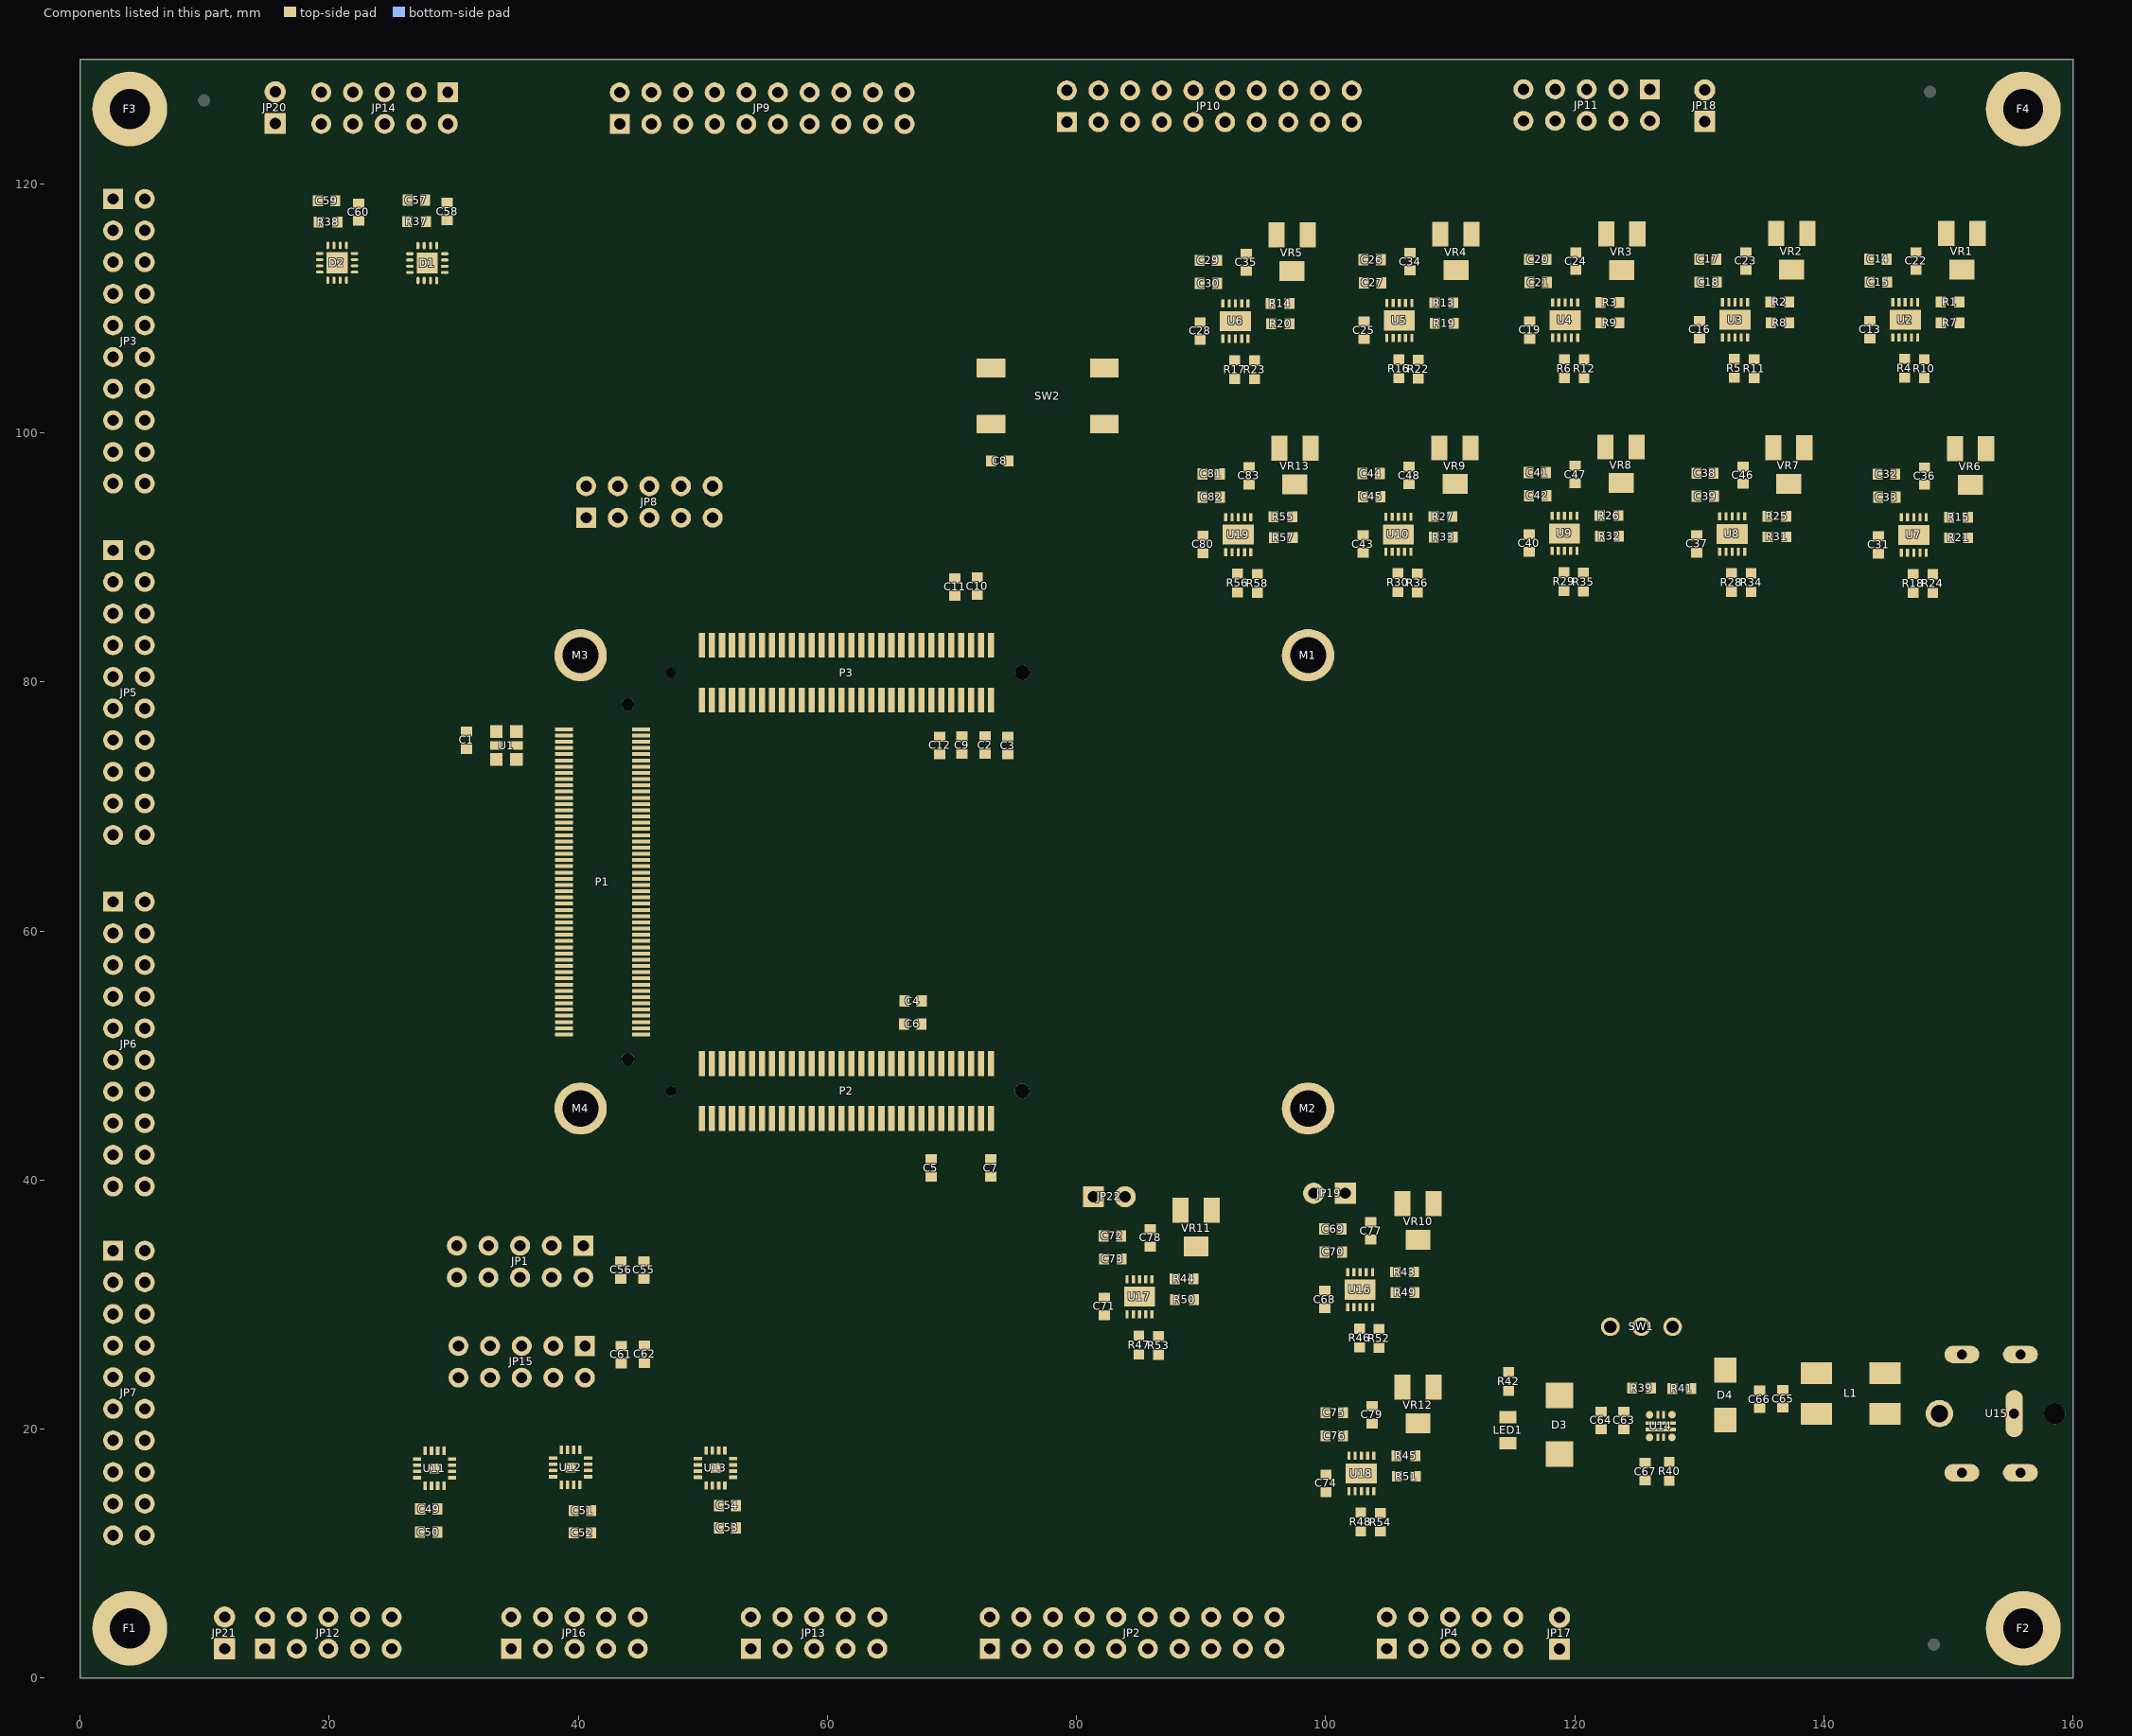
[diagram p0: the components of this part, seen from the top]
# Altium PCB MISC82195.PcbDoc (part 7 of 8)
Units mm, origin at the board's own origin, x right, y up, seen from the top; angles counter-clockwise.
Board outline 160 x 130 mm, 4 copper layers (Top Layer, GND, POWER, Bottom Layer); 214 components, 251 nets, 1068 pads, 1218 vias.

## Polygon pours and split planes (outlines as drawn) (continued)
VCC5VD on Top Layer "Bottom Layer-No Net" (solid, remove dead copper, pour order 1031): 113.081,17.374 113.081,14.199 113.411,13.868 114.071,13.208 115.316,13.208 122.58,13.208 123.038,13.665 123.723,14.351 123.723,16.891 123.723,17.323 124.79,18.39 125.095,18.694 125.095,19.228 125.095,19.38 125.298,19.583 125.527,19.812 125.806,19.812 128.092,19.812 128.143,19.863 128.168,19.888 128.168,19.964 128.168,20.117 128.143,20.142 127.991,20.142 125.552,20.142 125.451,20.244 125.273,20.422 124.333,20.422 120.802,20.422 120.421,20.041 119.736,19.355 118.389,19.355 113.767,19.355 113.411,18.999 113.106,18.694 113.106,17.475
NetC65_2 on Top Layer "Bottom Layer-No Net" (solid, remove dead copper, pour order 1030): 125.679,20.523 125.679,20.371 125.705,20.345 125.73,20.32 125.781,20.32 128.575,20.32 128.651,20.244 128.753,20.142 128.753,19.837 128.753,18.567 128.88,18.44 129.794,17.526 131.521,17.526 139.878,17.526 140.31,17.958 140.716,18.364 140.716,20.091 140.716,21.844 140.462,22.098 140.437,22.123 138.354,22.123 130.734,22.123 130.454,22.403 130.226,22.631 130.226,23.317 130.226,23.647 130.124,23.749 130.073,23.8 129.667,23.8 129.032,23.8 128.956,23.724 128.956,23.546 128.956,21.361 128.6,21.006 128.245,20.65 127.889,20.65 125.705,20.65 125.679,20.625 125.679,20.523
NetL1_2 on Top Layer "Bottom Layer-No Net" (solid, remove dead copper, pour order 1029): 143.561,25.654 143.561,23.749 143.612,23.698 143.84,23.47 144.602,23.47 146.279,23.47 146.634,23.825 147.269,24.46 148.869,24.46 152.248,24.46 152.984,23.724 153.67,23.038 153.67,21.463 153.67,18.313 153.568,18.212 152.857,17.501 150.571,17.501 149.479,17.501 149.098,17.12 148.742,16.764 148.742,15.748 148.742,13.97 149.2,13.513 149.606,13.106 151.105,13.106 156.134,13.106 156.642,13.614 157.226,14.199 157.226,18.948 157.226,28.55 156.439,29.337 156.286,29.489 152.984,29.489 144.932,29.489 144.145,28.702 143.561,28.118 143.561,25.679
NetL1_1 on Top Layer "Bottom Layer-No Net" (solid, remove dead copper, pour order 1028): 143.459,21.336 143.459,18.771 143.688,18.542 143.942,18.288 145.059,18.288 149.809,18.288 150.012,18.491 150.419,18.898 150.419,20.015 150.419,21.844 150.012,22.25 149.86,22.403 148.158,22.403 147.396,22.403 147.142,22.149 145.847,22.149 143.688,22.149 143.561,22.022 143.459,21.92 143.459,21.336
VCC1V8D on Top Layer "Bottom Layer-No Net" (solid, remove dead copper, pour order 1027): 100.99,20.803 100.99,17.863 101.346,17.548 101.371,17.526 101.905,17.526 102.413,17.526 102.464,17.571 102.489,17.593 102.489,17.75 102.489,22.15 102.286,22.33 102.26,22.352 101.93,22.352 101.321,22.352 101.117,22.172 100.99,22.06 100.99,20.826
VCC5VD on Top Layer "Bottom Layer-No Net" (solid, remove dead copper, pour order 1026): 99.212,14.58 99.212,11.582 99.568,11.227 99.974,10.82 100.686,10.82 102.972,10.82 103.124,10.973 103.429,11.278 103.429,11.506 103.429,12.09 103.276,12.243 103.048,12.243 102.21,12.243 102.057,12.395 101.905,12.548 101.905,12.903 101.905,13.894 102.006,13.995 102.133,14.122 102.286,14.122 102.641,14.122 102.768,14.249 102.997,14.478 102.997,14.859 102.997,15.24 102.921,15.316 102.895,15.342 102.794,15.342 99.67,15.342 99.492,15.164 99.212,14.884 99.212,14.554
VCC5VD on Top Layer "Bottom Layer-No Net" (solid, remove dead copper, pour order 1024): 99.111,29.337 99.111,26.34 99.466,25.984 99.873,25.578 100.584,25.578 102.87,25.578 103.022,25.73 103.327,26.035 103.327,26.264 103.327,26.848 103.175,27 102.946,27 102.108,27 101.956,27.153 101.803,27.305 101.803,27.661 101.803,28.651 101.905,28.753 102.032,28.88 102.184,28.88 102.54,28.88 102.667,29.007 102.895,29.235 102.895,29.616 102.895,29.997 102.819,30.074 102.794,30.099 102.692,30.099 99.568,30.099 99.39,29.921 99.111,29.642 99.111,29.312
VCC5VD on Top Layer "Bottom Layer-No Net" (solid, remove dead copper, pour order 1022): 81.407,28.778 81.407,25.781 81.763,25.425 82.169,25.019 82.88,25.019 85.166,25.019 85.319,25.171 85.623,25.476 85.623,25.705 85.623,26.289 85.471,26.441 85.242,26.441 84.404,26.441 84.252,26.594 84.099,26.746 84.099,27.102 84.099,28.092 84.201,28.194 84.328,28.321 84.48,28.321 84.836,28.321 84.963,28.448 85.192,28.677 85.192,29.058 85.192,29.439 85.115,29.515 85.09,29.54 84.988,29.54 81.864,29.54 81.686,29.362 81.407,29.083 81.407,28.753
VCC5VD on Top Layer "Bottom Layer-No Net" (solid, remove dead copper, pour order 1021): 143.561,89.941 143.561,86.944 143.916,86.589 144.323,86.182 145.034,86.182 147.32,86.182 147.472,86.335 147.777,86.639 147.777,86.868 147.777,87.452 147.625,87.605 147.396,87.605 146.558,87.605 146.406,87.757 146.253,87.909 146.253,88.265 146.253,89.256 146.355,89.357 146.482,89.484 146.634,89.484 146.99,89.484 147.117,89.611 147.345,89.84 147.345,90.221 147.345,90.602 147.269,90.678 147.244,90.703 147.142,90.703 144.018,90.703 143.84,90.526 143.561,90.246 143.561,89.916
LDO_6 on Top Layer "Bottom Layer-No Net" (solid, remove dead copper, pour order 1020): 145.339,96.165 145.339,93.224 145.694,92.91 145.72,92.888 146.253,92.888 146.761,92.888 146.812,92.933 146.837,92.955 146.837,93.112 146.837,97.512 146.634,97.691 146.609,97.714 146.279,97.714 145.669,97.714 145.466,97.534 145.339,97.422 145.339,96.187
VCC5VD on Top Layer "Bottom Layer-No Net" (solid, remove dead copper, pour order 1019): 128.981,90.018 128.981,87.02 129.337,86.665 129.743,86.258 130.454,86.258 132.74,86.258 132.893,86.411 133.198,86.716 133.198,86.944 133.198,87.528 133.045,87.681 132.817,87.681 131.978,87.681 131.826,87.833 131.674,87.986 131.674,88.341 131.674,89.332 131.775,89.433 131.902,89.56 132.055,89.56 132.41,89.56 132.537,89.687 132.766,89.916 132.766,90.297 132.766,90.678 132.69,90.754 132.664,90.78 132.563,90.78 129.438,90.78 129.261,90.602 128.981,90.322 128.981,89.992
LDO_7 on Top Layer "Bottom Layer-No Net" (solid, remove dead copper, pour order 1018): 130.759,96.241 130.759,93.301 131.115,92.986 131.14,92.964 131.674,92.964 132.182,92.964 132.232,93.009 132.258,93.031 132.258,93.188 132.258,97.588 132.055,97.768 132.029,97.79 131.699,97.79 131.089,97.79 130.886,97.61 130.759,97.498 130.759,96.264
VCC5VD on Top Layer "Bottom Layer-No Net" (solid, remove dead copper, pour order 1017): 115.519,90.068 115.519,87.071 115.875,86.716 116.281,86.309 116.992,86.309 119.278,86.309 119.431,86.462 119.736,86.766 119.736,86.995 119.736,87.579 119.583,87.732 119.355,87.732 118.516,87.732 118.364,87.884 118.212,88.036 118.212,88.392 118.212,89.383 118.313,89.484 118.44,89.611 118.593,89.611 118.948,89.611 119.075,89.738 119.304,89.967 119.304,90.348 119.304,90.729 119.228,90.805 119.202,90.83 119.101,90.83 115.976,90.83 115.799,90.653 115.519,90.373 115.519,90.043
LDO_8 on Top Layer "Bottom Layer-No Net" (solid, remove dead copper, pour order 1016): 117.297,96.292 117.297,93.351 117.653,93.037 117.678,93.015 118.212,93.015 118.72,93.015 118.77,93.06 118.796,93.082 118.796,93.239 118.796,97.639 118.593,97.818 118.567,97.841 118.237,97.841 117.627,97.841 117.424,97.661 117.297,97.549 117.297,96.314
VCC5VD on Top Layer "Bottom Layer-No Net" (solid, remove dead copper, pour order 1015): 102.184,89.992 102.184,86.995 102.54,86.639 102.946,86.233 103.657,86.233 105.943,86.233 106.096,86.385 106.401,86.69 106.401,86.919 106.401,87.503 106.248,87.655 106.02,87.655 105.181,87.655 105.029,87.808 104.877,87.96 104.877,88.316 104.877,89.306 104.978,89.408 105.105,89.535 105.258,89.535 105.613,89.535 105.74,89.662 105.969,89.891 105.969,90.272 105.969,90.653 105.893,90.729 105.867,90.754 105.766,90.754 102.641,90.754 102.464,90.576 102.184,90.297 102.184,89.967
LDO_9 on Top Layer "Bottom Layer-No Net" (solid, remove dead copper, pour order 1014): 103.962,96.216 103.962,93.275 104.318,92.961 104.343,92.939 104.877,92.939 105.385,92.939 105.435,92.983 105.461,93.006 105.461,93.163 105.461,97.563 105.258,97.742 105.232,97.765 104.902,97.765 104.292,97.765 104.089,97.585 103.962,97.473 103.962,96.238
VCC5VD on Top Layer "Bottom Layer-No Net" (solid, remove dead copper, pour order 1013): 89.332,89.967 89.332,86.97 89.687,86.614 90.094,86.208 90.805,86.208 93.091,86.208 93.243,86.36 93.548,86.665 93.548,86.893 93.548,87.478 93.396,87.63 93.167,87.63 92.329,87.63 92.177,87.782 92.024,87.935 92.024,88.29 92.024,89.281 92.126,89.383 92.253,89.51 92.405,89.51 92.761,89.51 92.888,89.637 93.116,89.865 93.116,90.246 93.116,90.627 93.04,90.703 93.015,90.729 92.913,90.729 89.789,90.729 89.611,90.551 89.332,90.272 89.332,89.941
LDO_10 on Top Layer "Bottom Layer-No Net" (solid, remove dead copper, pour order 1012): 91.11,96.19 91.11,93.25 91.465,92.936 91.491,92.913 92.024,92.913 92.532,92.913 92.583,92.958 92.608,92.981 92.608,93.138 92.608,97.537 92.405,97.717 92.38,97.739 92.05,97.739 91.44,97.739 91.237,97.56 91.11,97.447 91.11,96.213
LDO_1 on Top Layer "Bottom Layer-No Net" (solid, remove dead copper, pour order 1011): 144.653,113.437 144.653,110.496 145.009,110.182 145.034,110.16 145.567,110.16 146.075,110.16 146.126,110.205 146.152,110.227 146.152,110.384 146.152,114.784 145.948,114.963 145.923,114.986 145.593,114.986 144.983,114.986 144.78,114.806 144.653,114.694 144.653,113.459
VCC5VD on Top Layer "Bottom Layer-No Net" (solid, remove dead copper, pour order 1010): 142.875,107.213 142.875,104.216 143.231,103.861 143.637,103.454 144.348,103.454 146.634,103.454 146.787,103.607 147.091,103.911 147.091,104.14 147.091,104.724 146.939,104.877 146.71,104.877 145.872,104.877 145.72,105.029 145.567,105.181 145.567,105.537 145.567,106.528 145.669,106.629 145.796,106.756 145.948,106.756 146.304,106.756 146.431,106.883 146.66,107.112 146.66,107.493 146.66,107.874 146.583,107.95 146.558,107.975 146.456,107.975 143.332,107.975 143.154,107.798 142.875,107.518 142.875,107.188
LDO_2 on Top Layer "Bottom Layer-No Net" (solid, remove dead copper, pour order 1009): 130.988,113.437 130.988,110.496 131.343,110.182 131.369,110.16 131.902,110.16 132.41,110.16 132.461,110.205 132.486,110.227 132.486,110.384 132.486,114.784 132.283,114.963 132.258,114.986 131.928,114.986 131.318,114.986 131.115,114.806 130.988,114.694 130.988,113.459
VCC5VD on Top Layer "Bottom Layer-No Net" (solid, remove dead copper, pour order 1008): 129.21,107.213 129.21,104.216 129.565,103.861 129.972,103.454 130.683,103.454 132.969,103.454 133.121,103.607 133.426,103.911 133.426,104.14 133.426,104.724 133.274,104.877 133.045,104.877 132.207,104.877 132.055,105.029 131.902,105.181 131.902,105.537 131.902,106.528 132.004,106.629 132.131,106.756 132.283,106.756 132.639,106.756 132.766,106.883 132.994,107.112 132.994,107.493 132.994,107.874 132.918,107.95 132.893,107.975 132.791,107.975 129.667,107.975 129.489,107.798 129.21,107.518 129.21,107.188
LDO_3 on Top Layer "Bottom Layer-No Net" (solid, remove dead copper, pour order 1007): 117.348,113.412 117.348,110.471 117.704,110.157 117.729,110.134 118.262,110.134 118.77,110.134 118.821,110.179 118.847,110.202 118.847,110.359 118.847,114.758 118.643,114.938 118.618,114.96 118.288,114.96 117.678,114.96 117.475,114.781 117.348,114.669 117.348,113.434
VCC5VD on Top Layer "Bottom Layer-No Net" (solid, remove dead copper, pour order 1006): 115.57,107.188 115.57,104.191 115.926,103.835 116.332,103.429 117.043,103.429 119.329,103.429 119.482,103.581 119.786,103.886 119.786,104.115 119.786,104.699 119.634,104.851 119.405,104.851 118.567,104.851 118.415,105.004 118.262,105.156 118.262,105.512 118.262,106.502 118.364,106.604 118.491,106.731 118.643,106.731 118.999,106.731 119.126,106.858 119.355,107.086 119.355,107.467 119.355,107.848 119.278,107.925 119.253,107.95 119.151,107.95 116.027,107.95 115.849,107.772 115.57,107.493 115.57,107.163
VCC5VD on Top Layer "Bottom Layer-No Net" (solid, remove dead copper, pour order 1005): 102.26,107.163 102.26,104.165 102.616,103.81 103.022,103.403 103.734,103.403 106.02,103.403 106.172,103.556 106.477,103.861 106.477,104.089 106.477,104.673 106.324,104.826 106.096,104.826 105.258,104.826 105.105,104.978 104.953,105.131 104.953,105.486 104.953,106.477 105.054,106.578 105.181,106.705 105.334,106.705 105.689,106.705 105.816,106.832 106.045,107.061 106.045,107.442 106.045,107.823 105.969,107.899 105.943,107.925 105.842,107.925 102.718,107.925 102.54,107.747 102.26,107.467 102.26,107.137
LDO_4 on Top Layer "Bottom Layer-No Net" (solid, remove dead copper, pour order 1004): 104.038,113.386 104.038,110.446 104.394,110.131 104.419,110.109 104.953,110.109 105.461,110.109 105.512,110.154 105.537,110.176 105.537,110.333 105.537,114.733 105.334,114.913 105.308,114.935 104.978,114.935 104.369,114.935 104.165,114.755 104.038,114.643 104.038,113.409
LDO_5 on Top Layer "Bottom Layer-No Net" (solid, remove dead copper, pour order 1003): 90.881,113.335 90.881,110.395 91.237,110.081 91.262,110.058 91.796,110.058 92.304,110.058 92.354,110.103 92.38,110.126 92.38,110.283 92.38,114.682 92.177,114.862 92.151,114.884 91.821,114.884 91.211,114.884 91.008,114.705 90.881,114.592 90.881,113.358
VCC5VD on Top Layer "Bottom Layer-No Net" (solid, remove dead copper, pour order 1002): 89.103,107.112 89.103,104.115 89.459,103.759 89.865,103.353 90.576,103.353 92.862,103.353 93.015,103.505 93.32,103.81 93.32,104.038 93.32,104.623 93.167,104.775 92.939,104.775 92.1,104.775 91.948,104.927 91.796,105.08 91.796,105.435 91.796,106.426 91.897,106.528 92.024,106.655 92.177,106.655 92.532,106.655 92.659,106.782 92.888,107.01 92.888,107.391 92.888,107.772 92.812,107.848 92.786,107.874 92.685,107.874 89.56,107.874 89.383,107.696 89.103,107.417 89.103,107.086
NetJP8_1 on Top Layer "Bottom Layer-No Net" (solid, remove dead copper, pour order 1001): 39.675,93.116 39.675,90.246 40.157,89.764 40.843,89.078 43.231,89.078 46.431,89.078 47.142,88.367 49.505,86.004 49.505,83.058 49.505,82.067 49.555,82.017 49.682,81.89 49.809,81.89 52.476,81.89 52.502,81.915 52.578,81.991 52.578,82.423 52.578,93.116 51.968,93.726 51.664,94.031 50.622,94.031 39.878,94.031 39.776,93.929 39.675,93.828 39.675,93.116
NetJP1_1 on Top Layer "Bottom Layer-No Net" (solid, remove dead copper, pour order 1000): 29.388,35.331 29.388,34.671 29.388,34.265 29.667,33.985 29.921,33.731 31.14,33.731 41.427,33.731 42.443,34.747 45.314,37.617 47.244,37.617 49.327,37.617 50.546,38.837 52.578,40.869 52.578,44.044 52.578,45.847 52.502,45.923 52.426,45.999 51.943,45.999 49.733,45.999 49.657,45.923 49.301,45.568 49.301,44.806 49.301,44.044 48.158,42.901 47.142,41.885 46.101,41.885 45.364,41.885 43.942,40.462 40.284,36.805 34.011,36.805 30.683,36.805 29.413,35.535 29.388,35.509 29.388,35.331
VCC3V3D on Top Layer "Bottom Layer-No Net" (solid, remove dead copper, pour order 1000): 100.66,39.268 100.66,38.735 100.66,37.059 100.762,36.957 100.838,36.881 100.838,36.474 100.838,32.588 101.016,32.41 101.168,32.258 101.625,32.258 102.311,32.258 102.362,32.309 102.413,32.36 102.413,32.537 102.413,37.287 102.591,37.465 102.845,37.719 102.845,38.329 102.845,39.726 102.667,39.903 102.54,40.03 102.133,40.03 100.889,40.03 100.686,39.827 100.66,39.802 100.66,39.294
VCC2V5D on Top Layer "Bottom Layer-No Net" (solid, remove dead copper, pour order 1001): 83.007,38.76 83.007,36.347 83.134,36.22 83.185,36.17 83.185,35.89 83.185,32.004 83.388,31.801 83.464,31.725 83.998,31.725 84.607,31.725 84.658,31.775 84.684,31.801 84.684,31.902 84.684,32.537 84.785,32.639 84.912,32.766 84.912,32.944 84.912,39.243 84.658,39.497 84.531,39.624 84.328,39.624 83.337,39.624 83.134,39.421 83.007,39.294 83.007,38.76
GND on Bottom Layer "Bottom Layer-No Net" (solid, remove dead copper, pour order 1034): -7.925,128.981 -7.925,-4.267 -3.048,-9.144 -0.787,-11.405 6.325,-11.405 161.747,-11.405 165.506,-7.645 172.644,-0.508 172.644,18.237 172.644,132.74 165.887,139.497 160.63,144.755 147.853,144.755 2.184,144.755 -5.309,137.262 -8.306,134.264 -8.306,130.505
GND on GND (split plane): 159.49,0.51 0.51,0.51 0.51,129.49 159.49,129.49
VCC5VD on POWER (split plane): 159.49,0.51 26.164,0.51 26.164,12.01 28.376,14.222 54.047,14.222 54.048,14.221 54.101,14.18 54.163,14.154 54.229,14.146 54.295,14.154 54.357,14.18 54.41,14.221 54.411,14.222 102.895,14.222 102.962,14.231 103.023,14.256 103.077,14.297 104.778,15.999 104.819,16.052 104.845,16.113 104.853,16.18 104.853,22.25 104.845,22.317 104.837,22.335 104.819,22.378 104.778,22.432 101.934,25.276 101.88,25.317 101.819,25.343 101.752,25.351 75.62,25.351 69.547,31.424 69.547,50.237 71.201,51.89 75.484,51.89 78.916,48.459 78.916,38.227 78.924,38.161 78.95,38.099 78.991,38.046 80.947,36.089 80.957,36.067 80.997,36.014 81.05,35.973 81.112,35.948 81.178,35.939 93.04,35.939 93.107,35.948 93.168,35.973 93.221,36.014 93.983,36.776 94.024,36.829 94.05,36.891 94.058,36.957 94.058,40.813 94.747,41.501 99.817,41.501 100.252,41.067 100.252,37.744 100.26,37.678 100.286,37.616 100.327,37.563 101.444,36.446 101.497,36.405 101.559,36.379 101.625,36.371 115.062,36.371 115.128,36.379 115.19,36.405 115.243,36.446 116.64,37.843 116.681,37.896 116.699,37.939 116.706,37.957 116.715,38.024 116.715,80.315 116.706,80.381 116.688,80.425 116.681,80.443 116.64,80.496 114.43,82.706 114.377,82.746 114.316,82.772 114.249,82.781 89.616,82.781 86.972,85.425 86.972,91.664 88.498,93.19 94.412,93.19 94.478,93.199 94.54,93.225 94.593,93.265 95.812,94.485 95.853,94.538 95.878,94.599 95.887,94.666 95.887,100.711 95.878,100.777 95.866,100.808 95.853,100.839 95.812,100.892 94.161,102.543 94.108,102.584 94.046,102.609 93.98,102.618 89.159,102.618 87.429,104.348 87.429,129.49 159.49,129.49
LDO_10 on POWER (split plane): 86.917,104.242 86.925,104.175 86.951,104.114 86.992,104.06 88.871,102.181 88.924,102.14 88.986,102.115 89.052,102.106 93.874,102.106 95.375,100.605 95.375,94.772 94.306,93.703 88.392,93.703 88.326,93.694 88.264,93.668 88.211,93.628 86.609,92.026 74.274,92.026 58.525,107.776 58.472,107.816 58.41,107.842 58.344,107.851 22.733,107.851 22.667,107.842 22.605,107.816 22.552,107.776 15.364,100.587 15.323,100.534 15.297,100.473 15.289,100.406 15.289,32.639 15.297,32.573 15.323,32.511 15.364,32.458 20.113,27.708 20.167,27.667 20.21,27.649 20.228,27.642 20.295,27.633 48.941,27.633 53.973,22.601 53.973,14.734 28.27,14.734 28.204,14.725 28.142,14.7 28.089,14.659 25.727,12.297 25.686,12.244 25.661,12.182 25.652,12.116 25.652,0.51 0.51,0.51 0.51,129.49 86.917,129.49
VCC3V3D on POWER (split plane): 73.987,91.589 74.04,91.548 74.102,91.523 74.168,91.514 86.459,91.514 86.459,85.319 86.468,85.252 86.494,85.191 86.534,85.137 89.328,82.343 89.382,82.303 89.443,82.277 89.51,82.268 114.143,82.268 116.203,80.209 116.203,38.13 114.956,36.883 101.732,36.883 100.764,37.851 100.764,41.173 100.755,41.24 100.73,41.301 100.689,41.355 100.286,41.758 101.603,43.075 101.644,43.128 101.662,43.172 101.67,43.19 101.678,43.256 101.678,49.784 101.67,49.85 101.662,49.868 101.644,49.912 101.603,49.965 73.738,77.83 73.738,84.201 73.73,84.267 73.712,84.311 73.704,84.329 73.663,84.382 71.809,86.236 71.756,86.277 71.694,86.303 71.628,86.311 50.906,86.311 44.782,92.435 44.782,97.968 44.774,98.034 44.756,98.078 44.748,98.096 44.707,98.149 42.523,100.333 42.47,100.374 42.408,100.4 42.342,100.408 38.532,100.408 38.465,100.4 38.404,100.374 38.351,100.333 36.344,98.327 36.303,98.274 36.278,98.212 36.269,98.146 36.269,28.145 20.401,28.145 15.801,32.745 15.801,100.3 22.839,107.338 58.238,107.338
VCC1V8D on POWER (split plane): 44.27,97.862 44.27,92.329 44.279,92.263 44.304,92.201 44.345,92.148 50.619,85.874 50.672,85.833 50.716,85.815 50.734,85.808 50.8,85.799 71.522,85.799 73.226,84.095 73.226,77.724 73.235,77.658 73.26,77.596 73.301,77.543 101.166,49.678 101.166,43.362 99.936,42.132 99.933,42.132 99.872,42.106 99.819,42.066 99.779,42.014 94.64,42.014 94.574,42.005 94.512,41.979 94.459,41.939 93.621,41.101 93.58,41.047 93.555,40.986 93.546,40.919 93.546,37.063 92.934,36.451 81.31,36.451 79.428,38.333 79.428,48.565 79.419,48.631 79.394,48.693 79.353,48.746 75.772,52.327 75.718,52.368 75.657,52.394 75.59,52.402 71.095,52.402 71.028,52.394 70.985,52.376 70.967,52.368 70.913,52.327 69.11,50.524 69.069,50.471 69.044,50.409 69.035,50.343 69.035,31.318 69.044,31.252 69.069,31.19 69.11,31.137 75.333,24.914 75.386,24.873 75.43,24.855 75.448,24.848 75.514,24.839 101.646,24.839 104.341,22.144 104.341,16.286 102.789,14.734 54.485,14.734 54.485,22.708 54.476,22.774 54.458,22.818 54.451,22.836 54.41,22.889 49.229,28.07 49.175,28.111 49.114,28.137 49.047,28.145 36.781,28.145 36.781,98.039 38.638,99.896 42.236,99.896

## Keep-outs
Keep-Out Layer:
  the board outline again, w0.127

## Other copper
POWER (plane layer: these items are gaps in the copper):
  lines w0.508: 25.908,0.483 25.908,12.116 28.27,14.478 102.895,14.478 104.597,16.18 104.597,22.25 101.752,25.095 81.28,25.095 ; 36.525,28.118 36.525,98.146 38.532,100.152 42.342,100.152 44.526,97.968 44.526,92.329 50.8,86.055 71.628,86.055 73.482,84.201 73.482,77.724 101.422,49.784 101.422,43.256 100.051,41.885 100,41.885 ; 54.229,14.402 54.229,22.708 49.047,27.889 20.295,27.889 15.545,32.639 15.545,100.406 22.733,107.594 58.344,107.594 74.168,91.77 86.716,91.77 ; 81.178,36.195 93.04,36.195 93.802,36.957 93.802,40.919 94.64,41.758 99.924,41.758 100.508,41.173 100.508,37.744 101.625,36.627 115.062,36.627 116.459,38.024 116.459,80.315 114.249,82.525 89.51,82.525 86.716,85.319 86.716,91.77 ; 81.432,36.195 81.204,36.195 79.172,38.227 79.172,48.565 75.59,52.146 71.095,52.146 69.291,50.343 69.291,31.318 75.514,25.095 81.509,25.095 ; 87.173,129.87 87.173,104.242 89.052,102.362 93.98,102.362 95.631,100.711 95.631,94.666 94.412,93.447 88.392,93.447 86.716,91.77